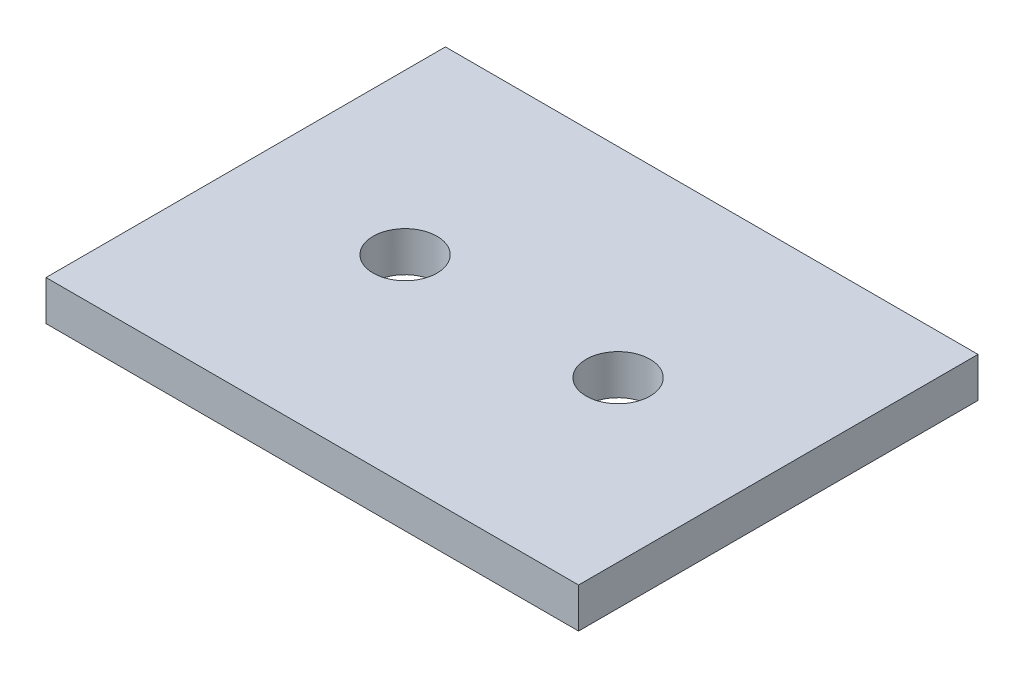
from build123d import *

# Parameters (mm, degrees)
SKETCH1_W                = 40
SKETCH1_H                = 30
BOSS_EXTRUDE1_DEPTH      = 3
M4_CLEARANCE_HOLE1_D     = 4.8
M4_CLEARANCE_HOLE1_DEPTH = 10.1
M4_CLEARANCE_HOLE1_TIP   = 1.442065486


with BuildPart() as part:
    # Sketch1 → Boss-Extrude1 (new body)
    with BuildSketch(Plane(origin=(0, 0, 0), x_dir=(1, 0, 0), z_dir=(0, 1, 0))):
        Rectangle(SKETCH1_W, SKETCH1_H)
    extrude(amount=BOSS_EXTRUDE1_DEPTH)

    # M4 Clearance Hole1
    with Locations(Plane(origin=(-8, 0, 0.030903026), x_dir=(0, 0, -1), z_dir=(0, -1, 0))):
        with Locations((0, 0), (0, 16)):
            Hole(M4_CLEARANCE_HOLE1_D / 2, depth=M4_CLEARANCE_HOLE1_DEPTH)
            with Locations((0, 0, -(M4_CLEARANCE_HOLE1_DEPTH + M4_CLEARANCE_HOLE1_TIP / 2))):  # 118° drill point
                Cone(0, M4_CLEARANCE_HOLE1_D / 2, M4_CLEARANCE_HOLE1_TIP, mode=Mode.SUBTRACT)


solid = part.part
